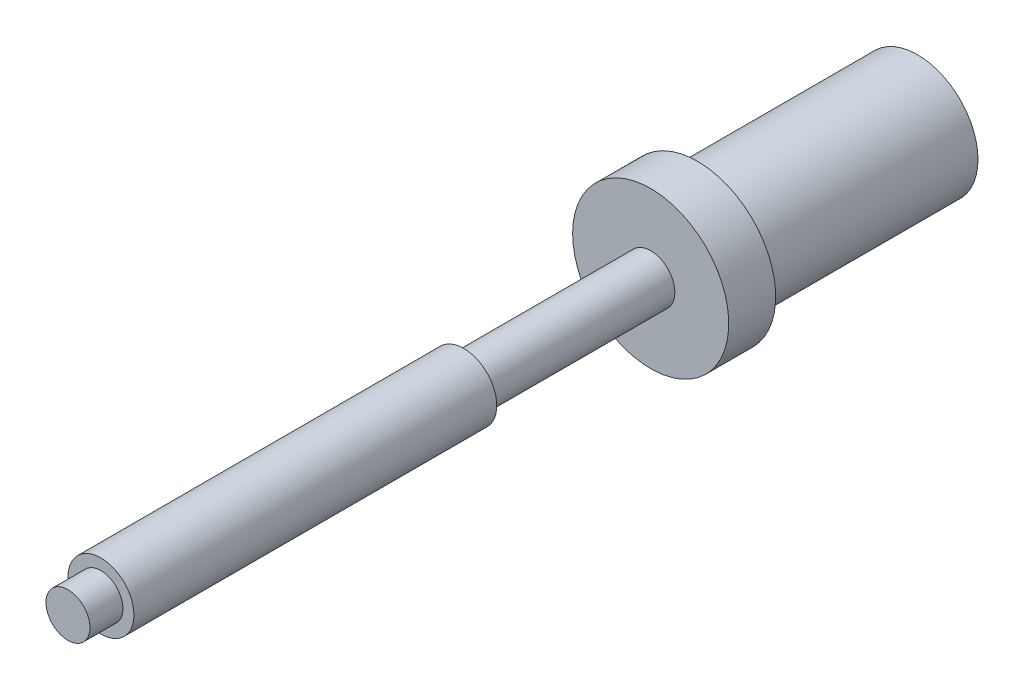
from build123d import *

# Parameters (mm, degrees)
SKETCH1_R           = 27.5
SKETCH1_R_2         = 17.5
BOSS_EXTRUDE1_DEPTH = 100
SKETCH2_R           = 35.5
BOSS_EXTRUDE2_DEPTH = 21.35
SKETCH3_R           = 11
BOSS_EXTRUDE3_DEPTH = 85
SKETCH4_R           = 15
BOSS_EXTRUDE4_DEPTH = 165
SKETCH5_R           = 10
BOSS_EXTRUDE5_DEPTH = 15


with BuildPart() as part:
    # Sketch1 → Boss-Extrude1 (new body)
    with BuildSketch(Plane.XY):
        Circle(SKETCH1_R)
        Circle(SKETCH1_R_2, mode=Mode.SUBTRACT)
    extrude(amount=BOSS_EXTRUDE1_DEPTH)

    # Sketch2 → Boss-Extrude2 (add)
    with BuildSketch(Plane.XY.offset(100)):
        with Locations(Location((0, 0, 0), (0, 0, 180))):
            Circle(SKETCH2_R)
    extrude(amount=BOSS_EXTRUDE2_DEPTH)

    # Sketch3 → Boss-Extrude3 (add)
    with BuildSketch(Plane.XY.offset(121.35)):
        Circle(SKETCH3_R)
    extrude(amount=BOSS_EXTRUDE3_DEPTH)

    # Sketch4 → Boss-Extrude4 (add)
    with BuildSketch(Plane.XY.offset(206.35)):
        Circle(SKETCH4_R)
    extrude(amount=BOSS_EXTRUDE4_DEPTH)

    # Sketch5 → Boss-Extrude5 (add)
    with BuildSketch(Plane.XY.offset(371.35)):
        Circle(SKETCH5_R)
    extrude(amount=BOSS_EXTRUDE5_DEPTH)


solid = part.part
